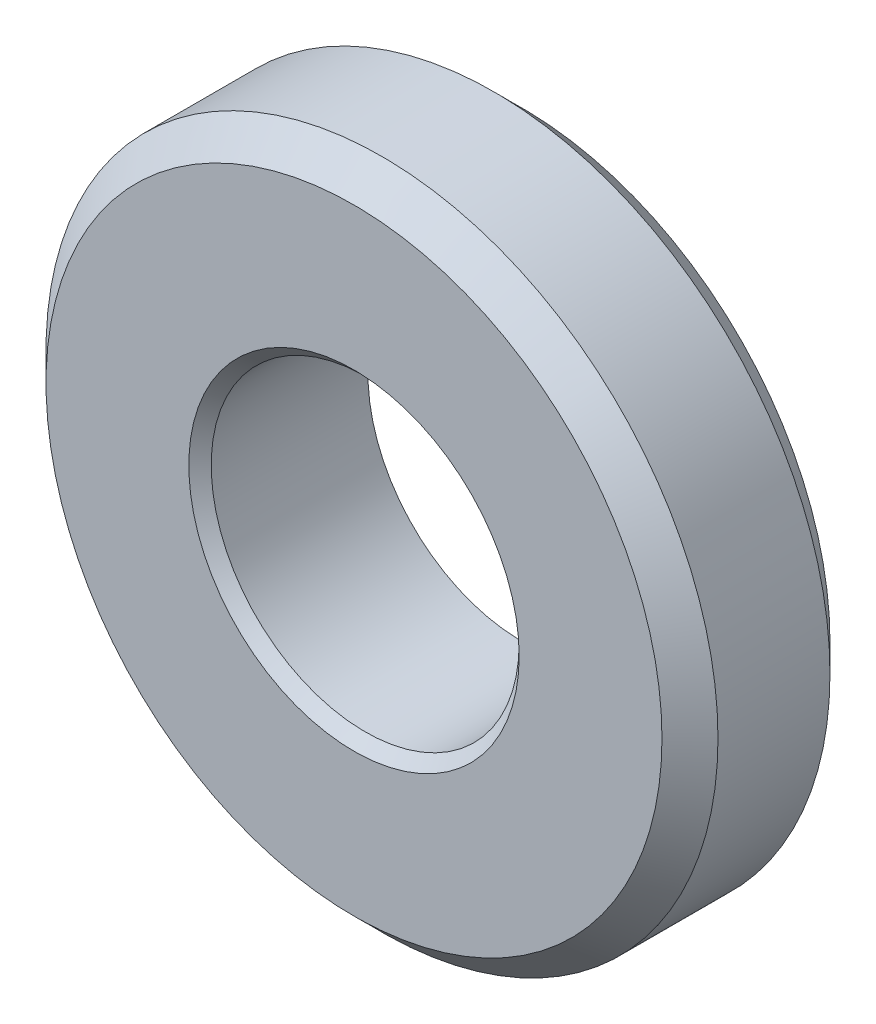
SolidWorks part; units mm, degrees
ref_plane "Front Plane" through (0, 0, 0) normal (0, 0, 1) x (1, 0, 0)
ref_plane "Top Plane" through (0, 0, 0) normal (0, 1, 0) x (1, 0, 0)
ref_plane "Right Plane" through (0, 0, 0) normal (1, 0, 0) x (0, 0, -1)
sketch "Sketch1" plane through (0, 0, 0) normal (0, 0, 1) x (1, 0, 0)
  circle A0 centre (0, 0) radius 27.5
  circle A1 centre (0, 0) radius 60
  dimension "D1" = 55
  dimension "D2" = 120
extrude "Boss-Extrude1" add sketch "Sketch1" along normal blind 30
chamfer "Chamfer1" distance 5 angle 45 2 edges at (60, 0, 0) (60, 0, 30)
chamfer "Chamfer2" distance 2 angle 45 1 edges at (27.5, 0, 30)
